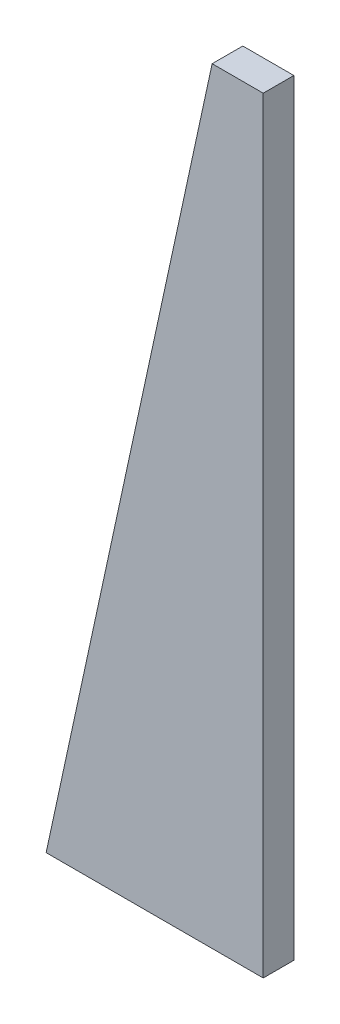
from build123d import *

# Parameters (mm, degrees)
EXTRUDE1_DEPTH = 6


with BuildPart() as part:
    # Sketch1 → Extrude1 (new, symmetric)
    with BuildSketch(Plane.XY):
        Polygon((0, 0), (0, 300), (-20, 300), (-85, 0), align=None)
    extrude(amount=EXTRUDE1_DEPTH, both=True)


solid = part.part
